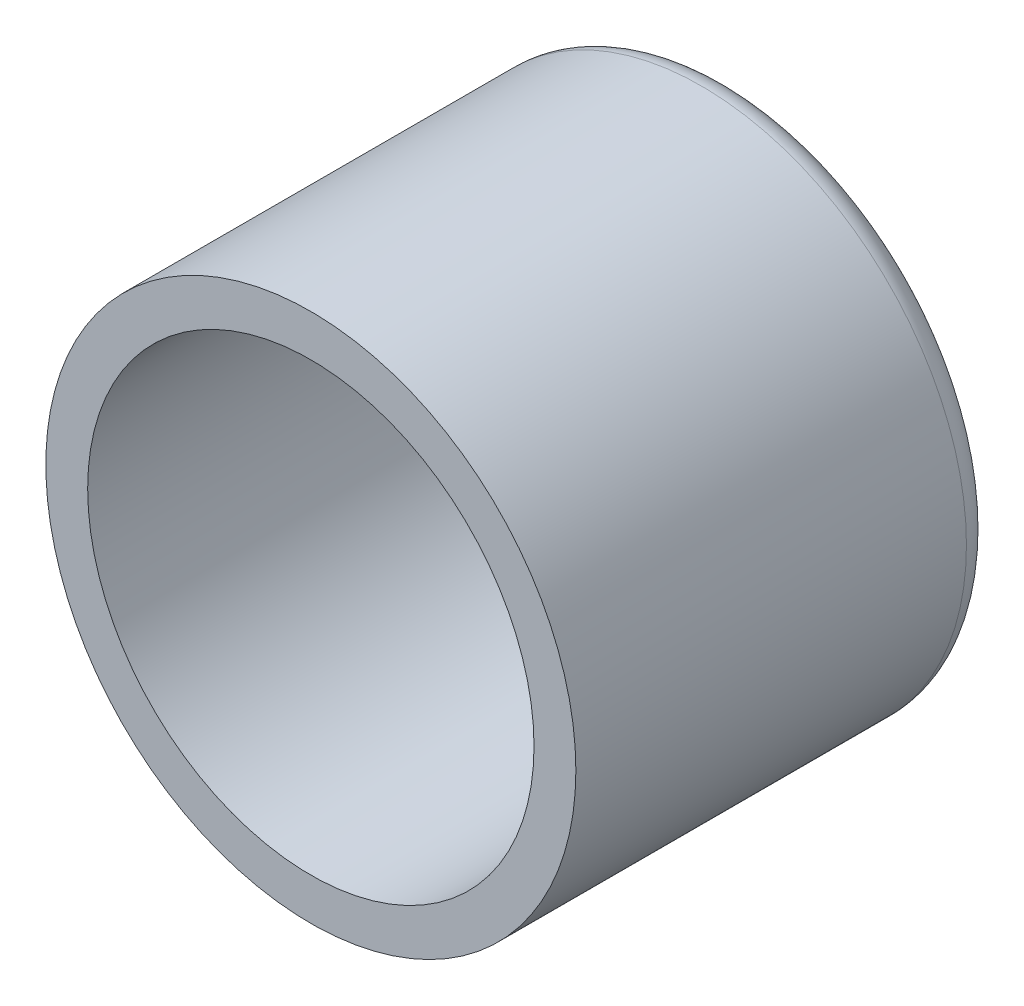
SolidWorks part; units mm, degrees
ref_plane "Front Plane" through (0, 0, 0) normal (0, 0, 1) x (1, 0, 0)
ref_plane "Top Plane" through (0, 0, 0) normal (0, 1, 0) x (1, 0, 0)
ref_plane "Right Plane" through (0, 0, 0) normal (1, 0, 0) x (0, 0, -1)
other "Configuration Table"
sketch "Sketch1" plane through (0, 0, 0) normal (0, 0, 1) x (1, 0, 0)
  circle A0 centre (-599.8842, -90) radius 80
  circle A1 centre (-599.8842, -90) radius 95
  dimension "D1" = 160
  dimension "D2" = 190
extrude "Boss-Extrude1" add sketch "Sketch1" along normal blind 100 and the other way blind 50
fillet "Fillet1" radius 10 1 edges at (-504.8842, -90, -50)
